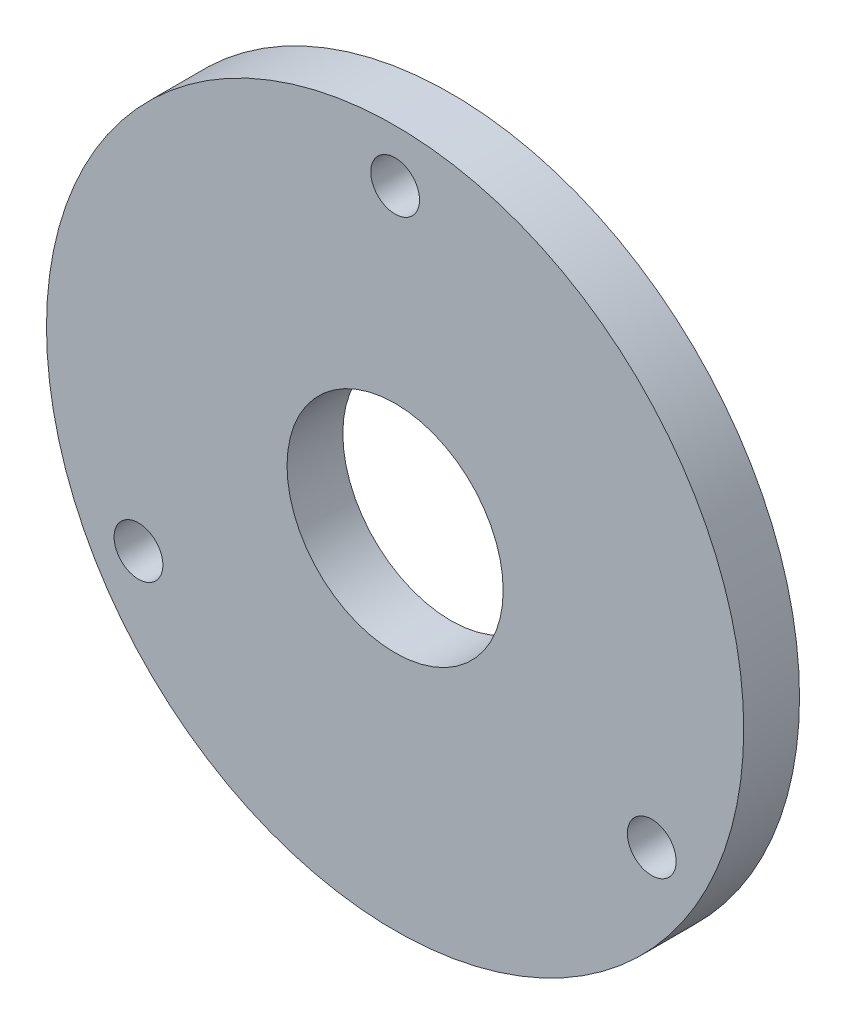
SolidWorks part; units mm, degrees
material "普通碳钢"
ref_plane "Front Plane" through (0, 0, 0) normal (0, 0, 1) x (1, 0, 0)
ref_plane "Top Plane" through (0, 0, 0) normal (0, 1, 0) x (1, 0, 0)
ref_plane "Right Plane" through (0, 0, 0) normal (1, 0, 0) x (0, 0, -1)
sketch "Sketch1" plane through (0, 0, 0) normal (0, 0, 1) x (1, 0, 0)
  line L0 (0, 42.5) -> (0, 0) construction
  line L1 (0, 0) -> (-36.8061, -21.25) construction
  line L2 (0, 0) -> (36.8061, -21.25) construction
  circle A0 centre (0, 0) radius 50
  circle A2 centre (0, 0) radius 42.5 construction
  circle A3 centre (0, 42.5) radius 3.5
  circle A4 centre (-36.8061, -21.25) radius 3.5
  circle A5 centre (36.8061, -21.25) radius 3.5
  circle A6 centre (0, 0) radius 15.5
  dimension "D1" = 100
  dimension "D2" = 85
  dimension "D3" = 7
  dimension "D6" = 31
  dimension "D4" = 120
  dimension "D5" = 120
extrude "Boss-Extrude1" add sketch "Sketch1" along normal blind 8
